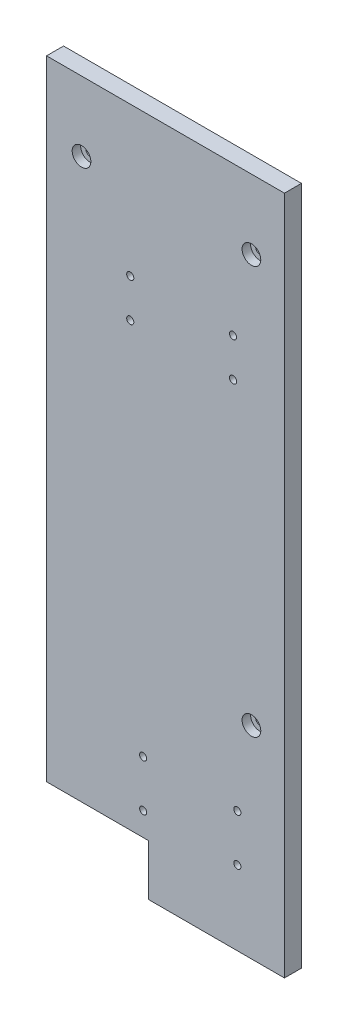
SolidWorks part; units mm, degrees
ref_plane "前视基准面" through (0, 0, 0) normal (0, 0, 1) x (1, 0, 0)
ref_plane "上视基准面" through (0, 0, 0) normal (0, 1, 0) x (1, 0, 0)
ref_plane "右视基准面" through (0, 0, 0) normal (1, 0, 0) x (0, 0, -1)
sketch "草图1" plane through (0, 0, 0) normal (0, 0, 1) x (1, 0, 0)
  line L0 (-99.5804, -70.7692) -> (-39.5804, -70.7692)
  line L1 (-39.5804, -70.7692) -> (-39.5804, -100.7692)
  line L2 (-39.5804, -100.7692) -> (40.4196, -100.7692)
  line L3 (40.4196, -100.7692) -> (40.4196, 299.2308)
  line L4 (40.4196, 299.2308) -> (-99.5804, 299.2308)
  line L5 (-99.5804, 299.2308) -> (-99.5804, -70.7692)
  dimension "D1" = 80
  dimension "D2" = 30
  dimension "D3" = 60
  dimension "D4" = 400
extrude "凸台-拉伸1" add sketch "草图1" along normal blind 10
sketch "草图10" plane through (0, 0, 10) normal (0, 0, 1) x (1, 0, 0)
  circle A0 centre (-79.0088, 258.253) radius 2.5
  circle A1 centre (20.9912, 258.253) radius 2.5
  circle A2 centre (-50.3304, 211.5825) radius 2.1
  circle A3 centre (-50.3304, 189.0825) radius 2.1
  circle A4 centre (10.1696, 211.5825) radius 2.1
  circle A5 centre (10.1696, 189.0825) radius 2.1
  circle A6 centre (-42.7171, -29.5192) radius 2.1
  circle A7 centre (-42.7171, -57.0192) radius 2.1
  circle A8 centre (12.7074, -57.0192) radius 2.1
  circle A9 centre (12.7074, -29.5192) radius 2.1
  circle A10 centre (20.9912, 18.253) radius 2.5
extrude "切除-拉伸1" cut sketch "草图10" against normal up to surface (10 mm away) up to face at (-32.9138, 42.5641, 0)
extrude "切除-拉伸2" cut sketch "草图11" against normal blind 5
sketch "草图11" plane through (-949.7244, 990.975, 10) normal (0, 0, 1) x (0, -1, 0)
  circle A1 centre (732.6808, 870.7156) radius 5.5
  circle A2 centre (732.722, 970.7156) radius 5.5
  circle A3 centre (972.722, 970.7156) radius 5.5
